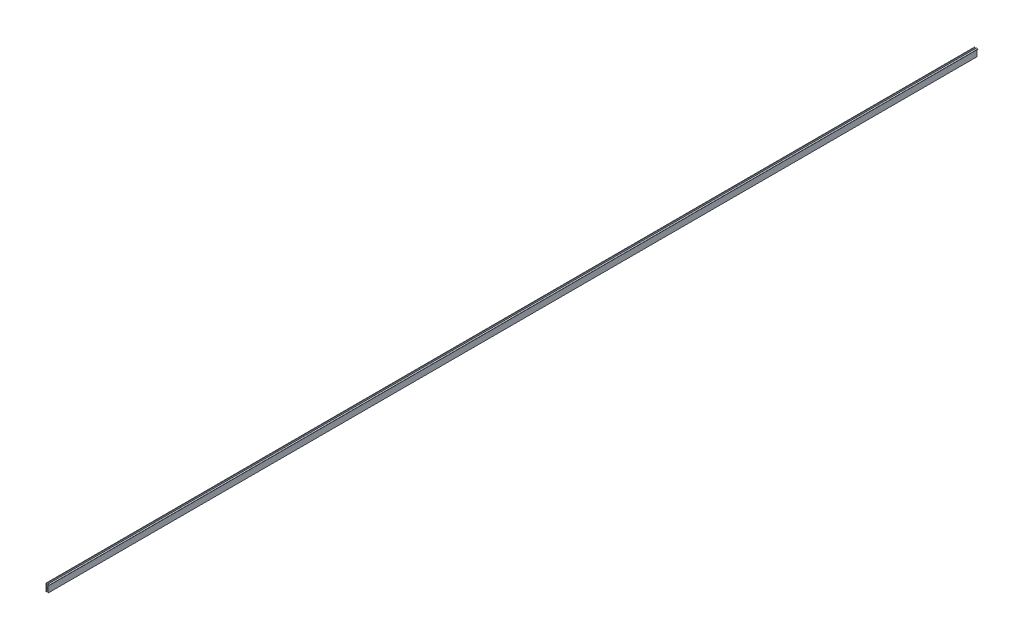
from build123d import *

# Parameters (mm, degrees)
EXTRUDE_1_DEPTH = 2317


with BuildPart() as part:
    # 草图1 → 凸台-拉伸1 (new body)
    with BuildSketch(Plane.XY):
        Polygon((7.255126662, 0), (3.255126662, 0), (3.255126662, -8.686153846), (-0.244873338, -8.686153846), (-0.244873338, 0), (-1.244873338, 0), (-1.244873338, -18.4), (-0.244873338, -18.4), (-0.244873338, -10.686153846), (3.255126662, -10.686153846), (3.255126662, -18.686153846), (4.255126662, -18.686153846), (4.255126662, -0.786153846), (7.255126662, -0.786153846), align=None)
    extrude(amount=EXTRUDE_1_DEPTH)


solid = part.part
